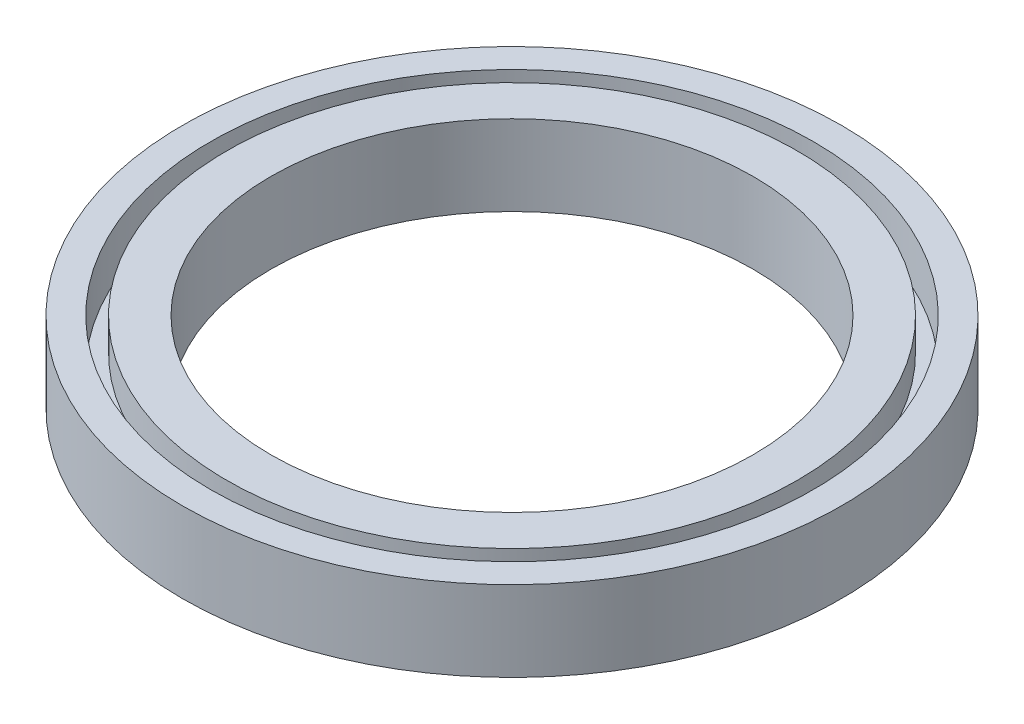
SolidWorks part; units mm, degrees
material "锰青铜"
ref_plane "前视基准面" through (0, 0, 0) normal (0, 0, 1) x (1, 0, 0)
ref_plane "上视基准面" through (0, 0, 0) normal (0, 1, 0) x (1, 0, 0)
ref_plane "右视基准面" through (0, 0, 0) normal (1, 0, 0) x (0, 0, -1)
other "Configuration Table"
sketch "草图1" plane through (0, 0, 0) normal (0, 1, 0) x (1, 0, 0)
  circle A0 centre (0, 0) radius 15
  circle A1 centre (0, 0) radius 20.5
  circle A2 centre (0, 0) radius 16.25
  circle A3 centre (0, 0) radius 18.75
  dimension "D1" = 30
  dimension "D2" = 41
  dimension "D3" = 32.5
  dimension "D4" = 37.5
extrude "凸台-拉伸1" add sketch "草图1" along normal blind 5 contours A2 A0 | A1 A3
sketch "草图2" plane through (0, 5, 0) normal (0, 1, 0) x (1, 0, 0)
  circle A0 centre (0, 0) radius 16.25
  circle A1 centre (0, 0) radius 16.25 construction
extrude "拉伸-薄壁1" add sketch "草图2" against normal blind 2 thin
sketch "草图3" plane through (0, 0, 0) normal (0, -1, 0) x (1, 0, 0)
  circle A0 centre (0, 0) radius 18.75
  circle A1 centre (0, 0) radius 18.75 construction
extrude "拉伸-薄壁2" add sketch "草图3" against normal blind 2 thin thin type one direction reverse wall 1.5
